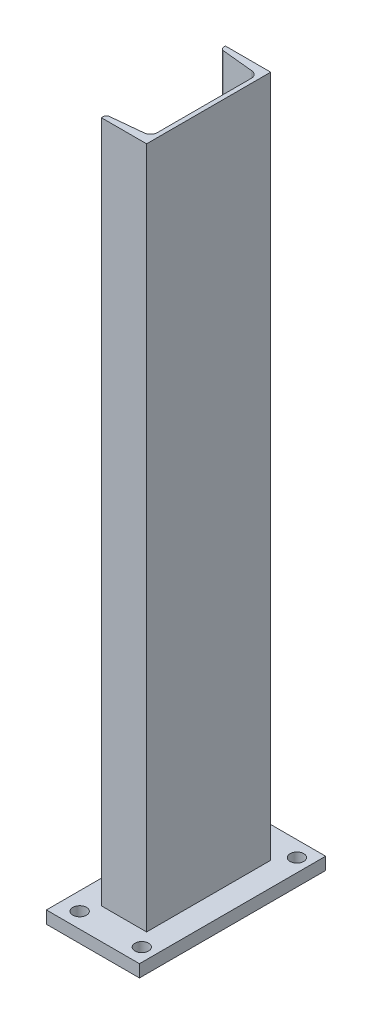
from build123d import *

# Parameters (mm, degrees)
STRUCTURAL_MEMBER1_DEPTH   = 1100
SKETCH3_W                  = 150
SKETCH3_H                  = 300
BOSS_EXTRUDE1_DEPTH        = 20
SKETCH4_W                  = 11
SKETCH4_H                  = 20.001
F_22_0_22_HOLE1_AT_2_COUNT = 2
F_22_0_22_HOLE1_AT_2_PITCH = 100
MIRROR1_COPY_1_SKETCH_W    = 11
MIRROR1_COPY_1_SKETCH_H    = 20.001


with BuildPart() as part:
    # Sketch1 → Structural Member1 (new body)
    with BuildSketch(Plane.XZ.offset(-588.709677419)):
        with BuildLine():
            Line((0, 0), (0, -200))
            Line((0, -200), (-73, -200))
            Line((-73, -200), (-73, -197.277431592))
            ThreePointArc((-73, -197.277431592), (-71.577988935, -193.586902327), (-68.047270455, -191.804727045))
            Line((-68.047270455, -191.804727045), (-16.905459091, -186.690545909))
            ThreePointArc((-16.905459091, -186.690545909), (-9.844022131, -183.126195345), (-7, -175.745136817))
            Line((-7, -175.745136817), (-7, -24.254863183))
            ThreePointArc((-7, -24.254863183), (-9.844022131, -16.873804655), (-16.905459091, -13.309454091))
            Line((-16.905459091, -13.309454091), (-68.047270455, -8.195272955))
            ThreePointArc((-68.047270455, -8.195272955), (-71.577988935, -6.413097673), (-73, -2.722568408))
            Line((-73, -2.722568408), (-73, 0))
            Line((-73, 0), (0, 0))
        make_face()
    extrude(amount=STRUCTURAL_MEMBER1_DEPTH)


with BuildPart() as body_2:
    # Sketch3 → Boss-Extrude1 (new body)
    with BuildSketch(Plane.XZ.offset(511.290322581)):
        with Locations((-36.5, -100)):
            Rectangle(SKETCH3_W, SKETCH3_H)
    extrude(amount=BOSS_EXTRUDE1_DEPTH)

    # Sketch4 → Ø22.0 (22) Hole1 (revolve, cut)
    with BuildSketch(Plane(origin=(-82.766539474, -511.290322581, -225), x_dir=(0, 0, 1), z_dir=(1, 0, 0))):
        with Locations((5.5, 10.0005)):
            Rectangle(SKETCH4_W, SKETCH4_H)
    f_22_0_22_hole1 = revolve(axis=Axis((-82.766539474, -504.940322581, -225), (0, -1, 0)), mode=Mode.SUBTRACT)

    # Ø22.0 (22) Hole1 at 2: Ø22.0 (22) Hole1 ×2
    with Locations(*[(i * F_22_0_22_HOLE1_AT_2_PITCH, 0, 0) for i in range(1, F_22_0_22_HOLE1_AT_2_COUNT)]):
        add(f_22_0_22_hole1, mode=Mode.SUBTRACT)

    # Mirror1: Ø22.0 (22) Hole1 across plane
    add(f_22_0_22_hole1.mirror(Plane(origin=(0, 0, -100), x_dir=(1, 0, 0), z_dir=(0, 0, -1))), mode=Mode.SUBTRACT)

    # Mirror1 copy 1 sketch → Mirror1 copy 1 (revolve, cut)
    with BuildSketch(Plane(origin=(17.233460526, -511.290322581, 25), x_dir=(0, 0, -1), z_dir=(1, 0, 0))):
        with Locations((5.5, -10.0005)):
            Rectangle(MIRROR1_COPY_1_SKETCH_W, MIRROR1_COPY_1_SKETCH_H)
    revolve(axis=Axis((17.233460526, -504.940322581, 25), (0, 1, 0)), mode=Mode.SUBTRACT)


solid = Compound([part.part, body_2.part])
